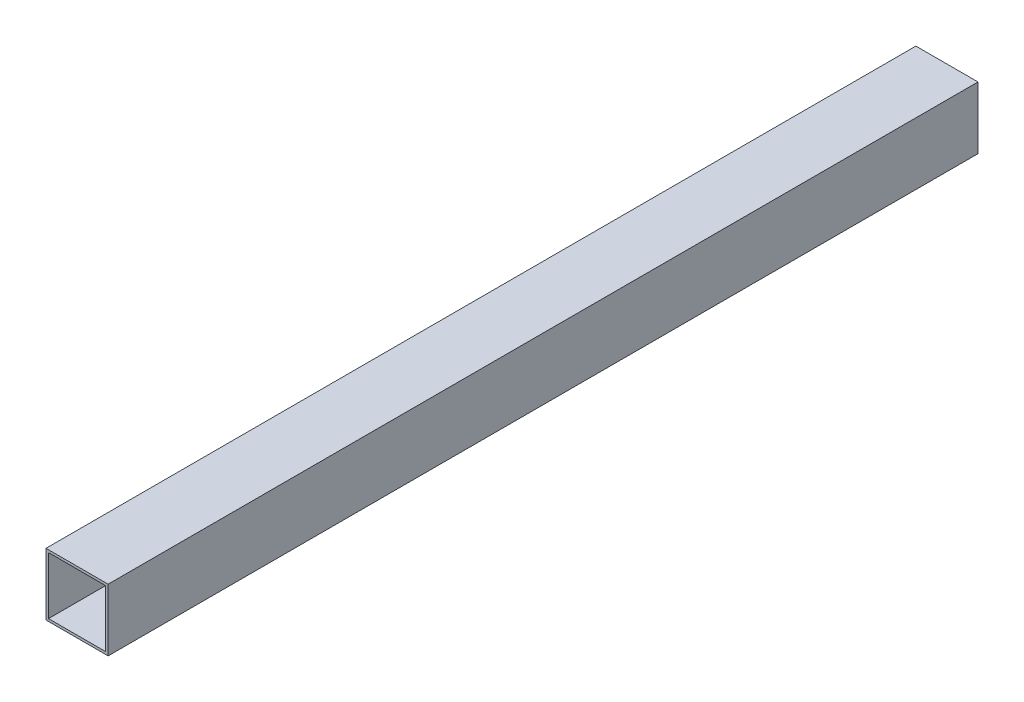
SolidWorks part; units mm, degrees
material "AISI 304"
ref_plane "Front Plane" through (0, 0, 0) normal (0, 0, 1) x (1, 0, 0)
ref_plane "Top Plane" through (0, 0, 0) normal (0, 1, 0) x (1, 0, 0)
ref_plane "Right Plane" through (0, 0, 0) normal (1, 0, 0) x (0, 0, -1)
sketch "Sketch1" plane through (0, 0, 0) normal (0, 0, 1) x (1, 0, 0)
  line L1 (-25, -25) -> (25, -25)
  line L2 (-25, -25) -> (-25, 25)
  line L3 (-25, 25) -> (25, 25)
  line L4 (25, -25) -> (25, 25)
  line L5 (-25, -25) -> (25, 25) construction
  line L6 (-25, 25) -> (25, -25) construction
  line L7 (-23, -23) -> (23, -23)
  line L8 (-23, -23) -> (-23, 23)
  line L9 (-23, 23) -> (23, 23)
  line L10 (23, -23) -> (23, 23)
  line L11 (-23, -23) -> (23, 23) construction
  line L12 (-23, 23) -> (23, -23) construction
  point P0 (0, 0)
  point P6 (0, 0)
  dimension "D1" = 50
  dimension "D2" = 50
  dimension "D3" = 46
  dimension "D4" = 46
extrude "Boss-Extrude1" add sketch "Sketch1" along normal blind 700
